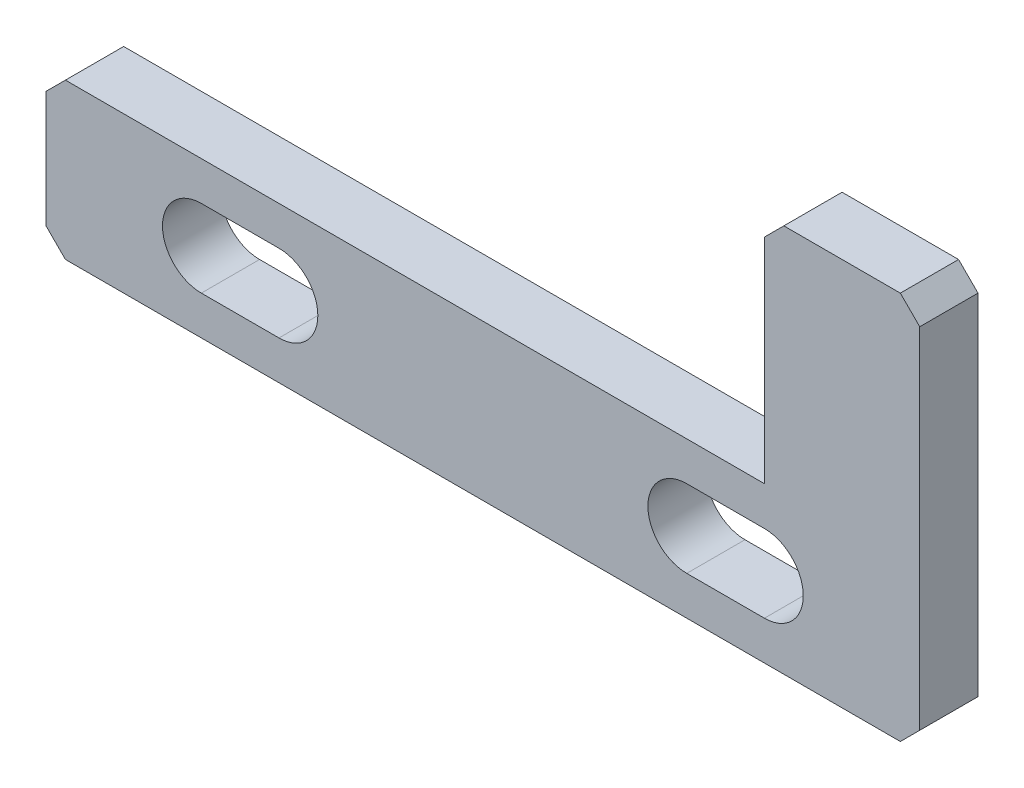
from build123d import *

# Parameters (mm, degrees)
BOSS_EXTRUDE1_DEPTH = 3
CUT_EXTRUDE1_DEPTH  = 3
CHAMFER1_SIZE       = 1


with BuildPart() as part:
    # Sketch1 → Boss-Extrude1 (new body)
    with BuildSketch(Plane.XY):
        Polygon((0, 0), (45, 0), (45, 20), (37, 20), (37, 8), (0, 8), align=None)
    extrude(amount=BOSS_EXTRUDE1_DEPTH)

    # Sketch2 → Cut-Extrude1 (cut)
    with BuildSketch(Plane(origin=(0, 0, 0), x_dir=(-1, 0, 0), z_dir=(0, 0, -1))):
        with BuildLine():
            Line((-37, 6), (-33, 6))
            ThreePointArc((-33, 6), (-31, 4), (-33, 2))
            Line((-33, 2), (-37, 2))
            ThreePointArc((-37, 2), (-39, 4), (-37, 6))
        make_face()
        with BuildLine():
            Line((-12, 6), (-8, 6))
            ThreePointArc((-8, 6), (-6, 4), (-8, 2))
            Line((-8, 2), (-12, 2))
            ThreePointArc((-12, 2), (-14, 4), (-12, 6))
        make_face()
    extrude(amount=-CUT_EXTRUDE1_DEPTH, mode=Mode.SUBTRACT)

    # Chamfer1
    chamfer1_edges = [part.edges().sort_by_distance(p)[0] for p in [
        (0, 8, 1.5),
        (37, 20, 1.5),
        (45, 20, 1.5),
        (45, 0, 1.5),
        (0, 0, 1.5),
    ]]
    chamfer(chamfer1_edges, length=CHAMFER1_SIZE)


solid = part.part
